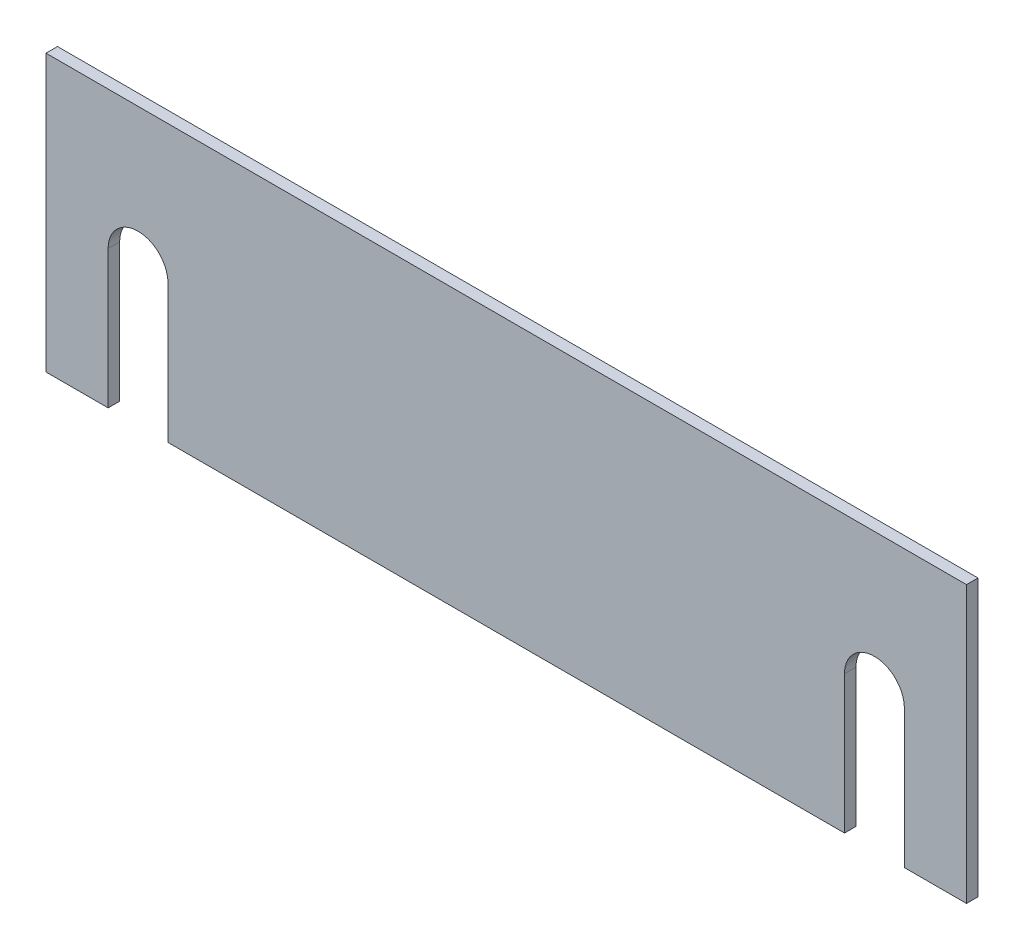
SolidWorks part; units mm, degrees
ref_plane "Front Plane" through (0, 0, 0) normal (0, 0, 1) x (1, 0, 0)
ref_plane "Top Plane" through (0, 0, 0) normal (0, 1, 0) x (1, 0, 0)
ref_plane "Right Plane" through (0, 0, 0) normal (1, 0, 0) x (0, 0, -1)
sketch "Sketch1" plane through (0, 0, 0) normal (0, 0, 1) x (1, 0, 0)
  line L1 (-200, 60) -> (200, 60)
  line L2 (-200, 60) -> (-200, -60)
  line L3 (-200, -60) -> (200, -60)
  line L4 (200, 60) -> (200, -60)
  line L5 (-200, 60) -> (200, -60) construction
  line L6 (-200, -60) -> (200, 60) construction
  point P0 (0, 0)
  dimension "D1" = 400
  dimension "D2" = 120
extrude "Boss-Extrude1" add sketch "Sketch1" along normal blind 5
sketch "Sketch2" plane through (0, 0, 5) normal (0, 0, 1) x (1, 0, 0)
  line L0 (0, 0) -> (0, 86.8425) construction
  line L1 (-160, 0) -> (-160, -96.9268) construction
  line L2 (-147, 0) -> (-147, -96.9268)
  line L3 (-173, 0) -> (-173, -96.9268)
  line L4 (-200, 60) -> (-200, -60) construction
  line L5 (-200, -60) -> (200, -60) construction
  line L6 (160, 0) -> (160, -96.9268) construction
  line L7 (147, 0) -> (147, -96.9268)
  line L8 (173, 0) -> (173, -96.9268)
  arc A0 (-147, 0) -> (-173, 0) centre (-160, 0) ccw
  arc A1 (-173, -96.9268) -> (-147, -96.9268) centre (-160, -96.9268) ccw
  arc A2 (147, 0) -> (173, 0) centre (160, 0) cw
  arc A3 (173, -96.9268) -> (147, -96.9268) centre (160, -96.9268) cw
  point P5 (-160, -48.4634)
  point P16 (160, -48.4634)
  dimension "D1" = 13
  dimension "D2" = 40
  dimension "D3" = 60
extrude "Cut-Extrude1" cut sketch "Sketch2" against normal through all
